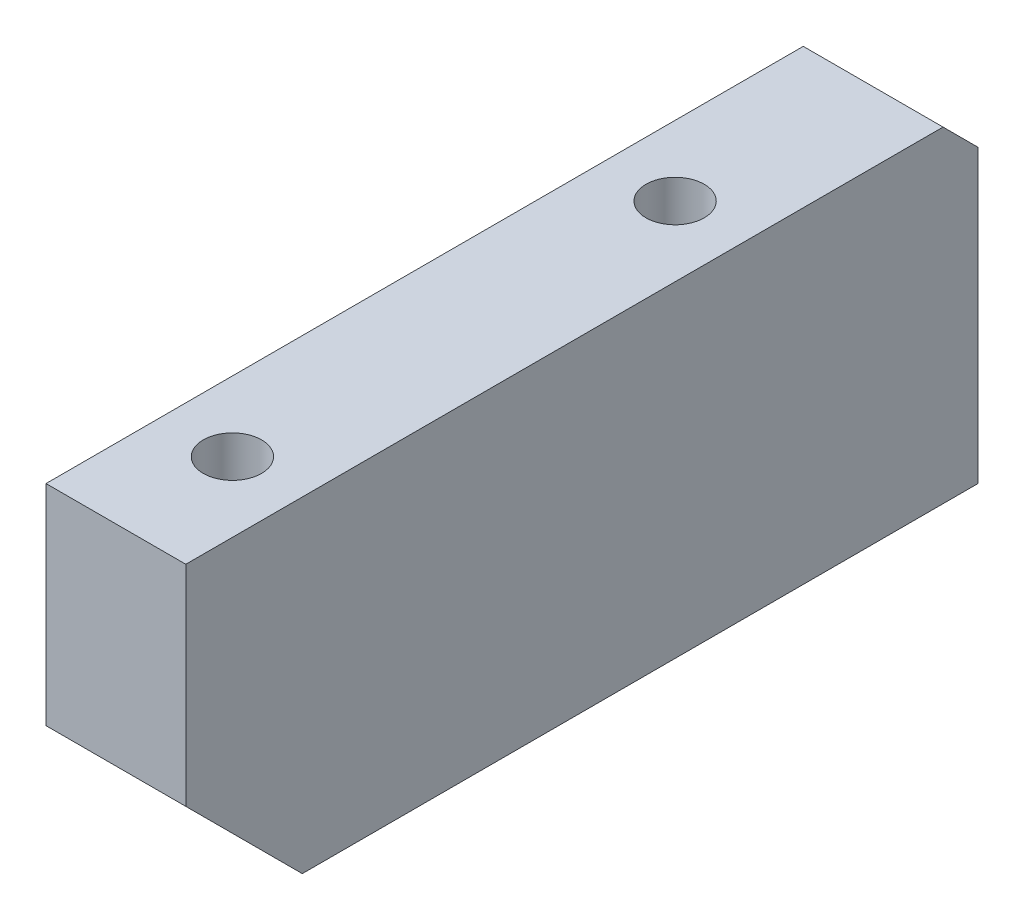
SolidWorks part; units mm, degrees
material "6061-T6 (SS)"
ref_plane "前视基准面" through (0, 0, 0) normal (0, 0, 1) x (1, 0, 0)
ref_plane "上视基准面" through (0, 0, 0) normal (0, 1, 0) x (1, 0, 0)
ref_plane "右视基准面" through (0, 0, 0) normal (1, 0, 0) x (0, 0, -1)
sketch "草图1" plane through (0, 0, 0) normal (0, 0, 1) x (1, 0, 0)
  line L1 (-250.9557, 0) -> (-238.9557, 0)
  line L2 (-250.9557, 0) -> (-250.9557, -28)
  line L3 (-250.9557, -28) -> (-238.9557, -28)
  line L4 (-238.9557, 0) -> (-238.9557, -28)
  dimension "D1" = 12
extrude "凸台-拉伸1" add sketch "草图1" along normal blind 68
chamfer "倒角1" distance 10 angle 45 1 edges at (-244.9557, -28, 68)
chamfer "倒角2" distance 3 angle 45 1 edges at (-244.9557, 0, 0)
hole_wizard "M6 螺纹孔1" positions "草图4" profile "草图2" tap size "M6" standard "Iso"
sketch "草图4" plane through (0, 0, 0) normal (0, 0, -1) x (-1, 0, 0)
  line L0 (238.9557, 0) -> (250.9557, 0) construction
  line L1 (238.9557, -28) -> (238.9557, -3) construction
  point P0 (244.9557, -9)
  point P6 (244.9557, -21)
  dimension "D1" = 9
  dimension "D2" = 12
  dimension "D3" = 6
sketch "草图2" plane through (-244.9557, -9, 0) normal (1, 0, 0) x (0, 1, 0)
  line L0 (0, 0) -> (0, 14.5022)
  line L1 (0, 14.5022) -> (2.5, 13)
  line L2 (2.5, 13) -> (2.5, 0)
  line L5 (2.5, 0) -> (0, 0)
  line L10 (0, 14.5022) -> (-2.5, 13) construction
  line L11 (0, -6.35) -> (0, 107.95) construction
  dimension "螺纹孔钻头直径" = 5
  dimension "螺纹孔钻头深度" = 13
  dimension "导头角度" = 118
cosmetic thread "孔螺蚊线1" parameters "D1"=12, "D2"=6
cosmetic thread "孔螺蚊线2" parameters "D1"=12, "D2"=6
hole_wizard "M6 螺纹孔2" positions "草图6" profile "草图5" tap size "M6" standard "Iso"
sketch "草图6" plane through (0, 0, 0) normal (0, 1, 0) x (1, 0, 0)
  line L0 (-250.9557, 0) -> (-238.9557, 0) construction
  line L1 (-238.9557, -68) -> (-250.9557, -68) construction
  line L2 (-250.9557, -68) -> (-250.9557, -3) construction
  point P0 (-244.9557, -58)
  point P2 (-244.9557, -20)
  dimension "D1" = 20
  dimension "D2" = 10
  dimension "D3" = 6
sketch "草图5" plane through (-244.9557, 0, 58) normal (1, 0, 0) x (0, 0, 1)
  line L0 (0, 0) -> (0, 14.5022)
  line L1 (0, 14.5022) -> (2.5, 13)
  line L2 (2.5, 13) -> (2.5, 0)
  line L5 (2.5, 0) -> (0, 0)
  line L10 (0, 14.5022) -> (-2.5, 13) construction
  line L11 (0, -6.35) -> (0, 107.95) construction
  dimension "螺纹孔钻头直径" = 5
  dimension "螺纹孔钻头深度" = 13
  dimension "导头角度" = 118
cosmetic thread "孔螺蚊线3" parameters "D1"=12, "D2"=6
cosmetic thread "孔螺蚊线4" parameters "D1"=12, "D2"=6
